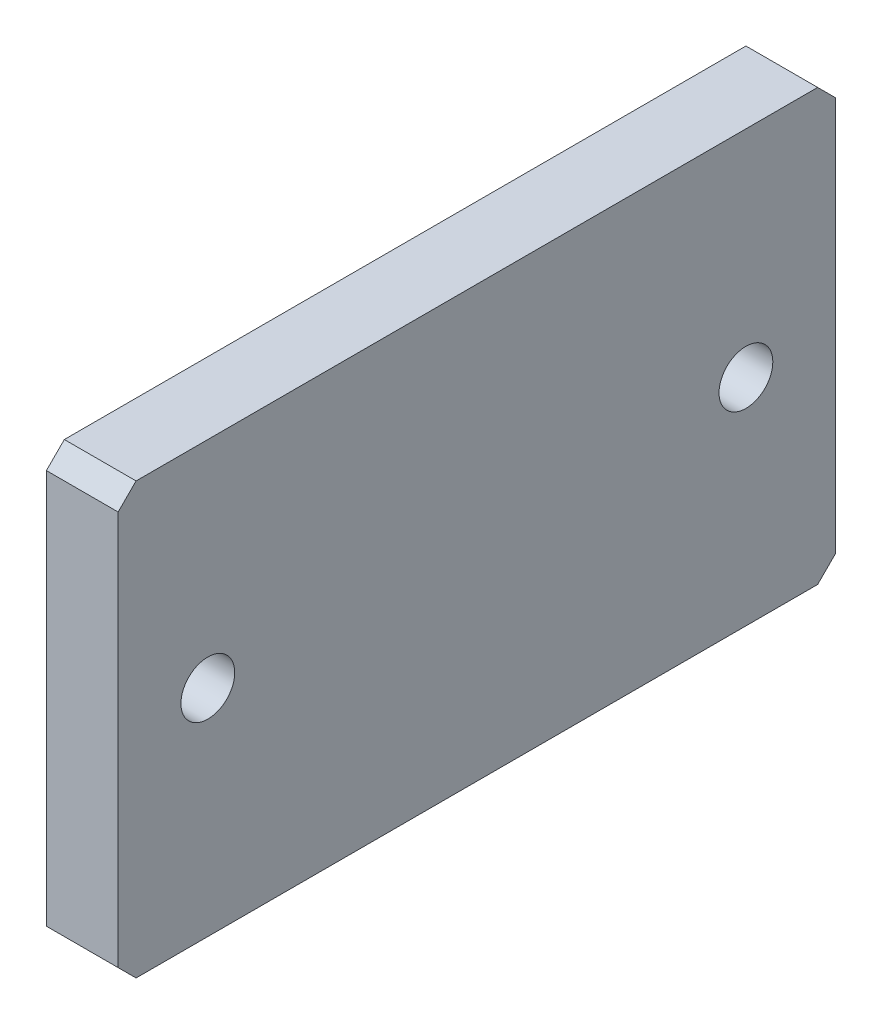
SolidWorks part; units mm, degrees
ref_plane "前视基准面" through (0, 0, 0) normal (0, 0, 1) x (1, 0, 0)
ref_plane "上视基准面" through (0, 0, 0) normal (0, 1, 0) x (1, 0, 0)
ref_plane "右视基准面" through (0, 0, 0) normal (1, 0, 0) x (0, 0, -1)
sketch "草图1" plane through (0, 0, 0) normal (1, 0, 0) x (0, 0, -1)
  line L1 (-100, 60) -> (100, 60)
  line L2 (-100, 60) -> (-100, -60)
  line L3 (-100, -60) -> (100, -60)
  line L4 (100, 60) -> (100, -60)
  line L5 (-100, 60) -> (100, -60) construction
  line L6 (-100, -60) -> (100, 60) construction
  point P0 (0, 0)
  dimension "D1" = 200
  dimension "D2" = 120
extrude "凸台-拉伸1" add sketch "草图1" along normal blind 20
hole_wizard "Ø15.0 (15) 直径孔1" positions "草图2" profile "草图3" hole size "Ø15.0" standard "GB" end condition through all
sketch "草图2" plane through (20, 0, 0) normal (1, 0, 0) x (0, 0, -1)
  line L0 (0, 0) -> (0, 64.4787) construction
  point P0 (-75, 0)
  point P2 (75, 0)
  dimension "D1" = 150
sketch "草图3" plane through (20, 0, 75) normal (0, 1, 0) x (0, 0, -1)
  line L0 (0, 0) -> (0, 20)
  line L1 (0, 20) -> (7.5, 20)
  line L2 (7.5, 20) -> (7.5, 0)
  line L5 (7.5, 0) -> (0, 0)
  line L11 (0, -6.35) -> (0, 107.95) construction
  dimension "通孔孔直径" = 15
  dimension "通孔孔深度" = 20
chamfer "倒角1" distance 5 angle 45 4 edges at (10, 60, 100) (10, -60, 100) (10, 60, -100) (10, -60, -100)
